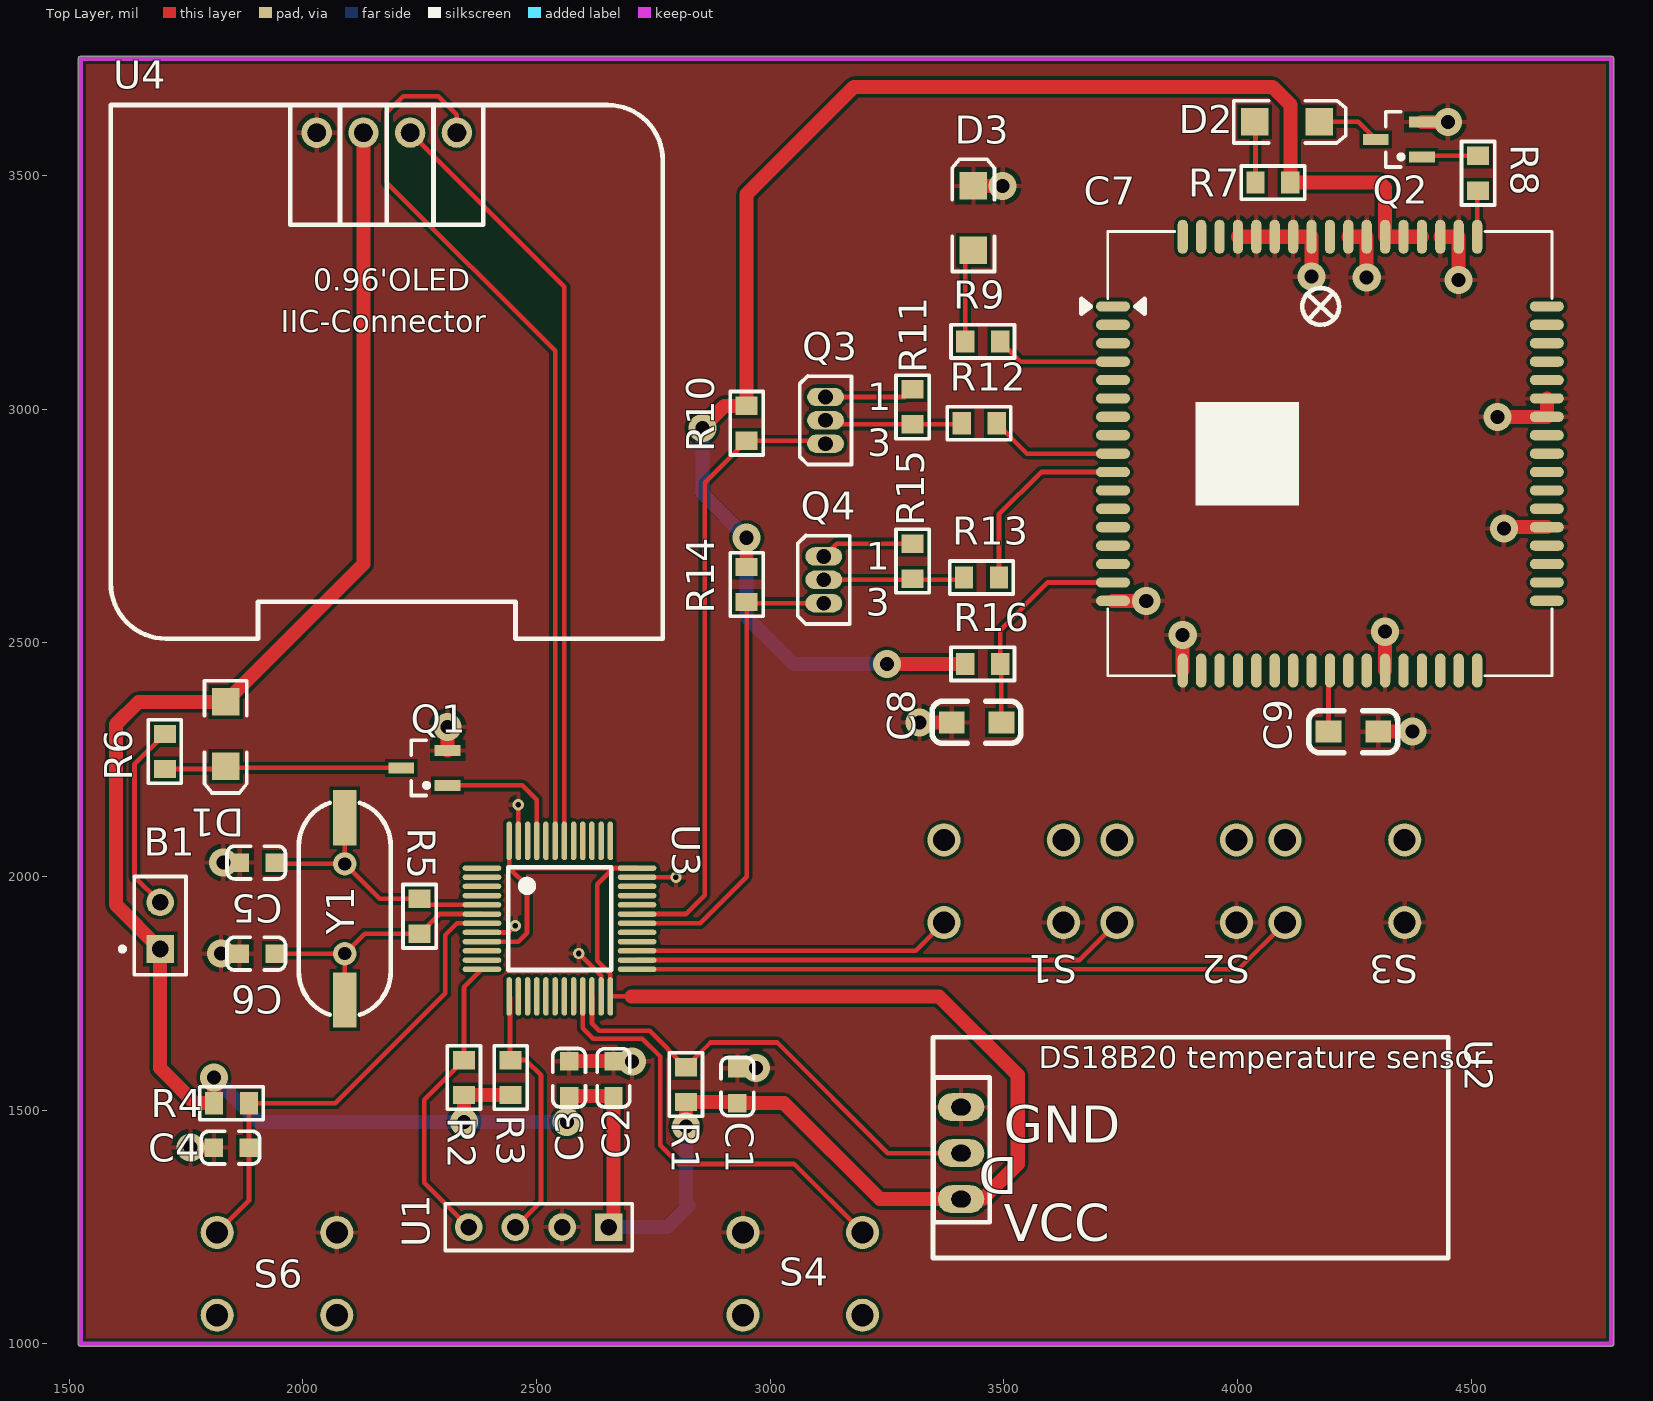
[diagram p0: Top Layer view]
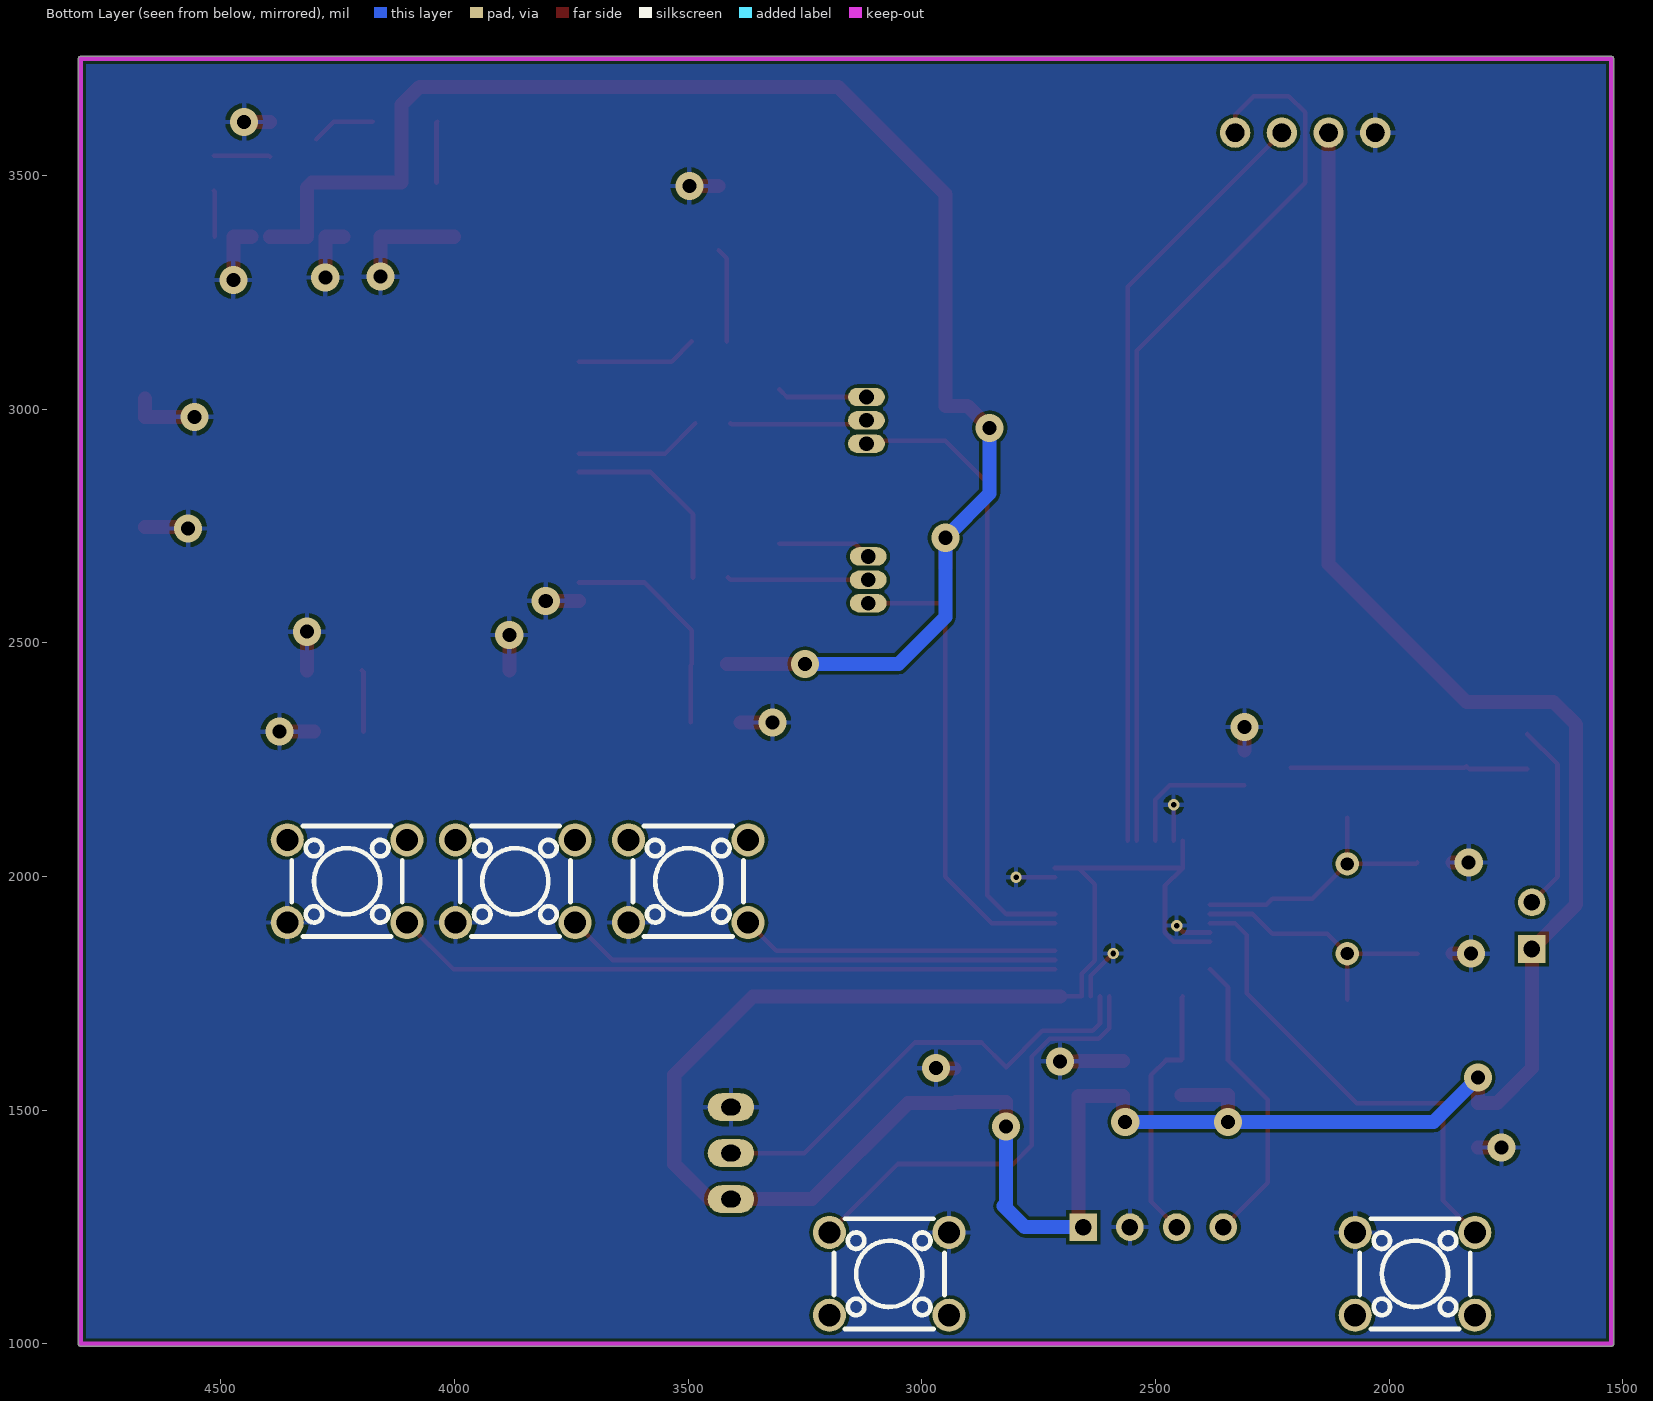
[diagram p1: Bottom Layer view, seen from below]
# Altium PCB MISC82701.PcbDoc
Units mil, origin at the board's own origin, x right, y up, seen from the top; angles counter-clockwise.
Board outline 3285.03 x 2760.03 mil, 2 copper layers (Top Layer, Bottom Layer); 43 components, 37 nets, 219 pads, 29 vias.

## Layer stack, top to bottom (the 12.6 mil dielectric is the usual default, probably not edited)
Top Solder: solder mask 0.4, Solder Resist, Dk 3.5
Top Layer: signal copper 1.4
Dielectric 1: dielectric 12.6, FR-4, Dk 4.8
Bottom Layer: signal copper 1.4
Bottom Solder: solder mask 0.4, Solder Resist, Dk 3.5

## Board outline
1519.98,1000 ccw(c1525,1000) 1525,994.99 4800,994.99 ccw(c4800,1000) 4805.02,1000 4805.02,3750 ccw(c4800,3750) 4800,3755.01 1525,3755.01 ccw(c1525,3750) 1519.98,3750

## Design rules (kind name [scope] priority, off if disabled: settings)
Clearance [All] p1: gap=7
MinimumSolderMaskSliver [All] p1: minsoldermaskwidth=0
PolygonConnect [All] p1: connectstyle=Relief reliefconductorwidth=10 reliefentries=4 polygonreliefangle="90 Angle" airgapwidth=10
RoutingVias [All] p1: holewidth=28 width=50 viastyle="Through Hole" minholewidth=28 minwidth=50 maxholewidth=28 maxwidth=50
SilkToSilkClearance [All] p1: silktosilkclearance=0
SilkToSolderMaskClearance [IsPad] p1: minsilkscreentomaskgap=0 clearancetoexposedcopper=TRUE
SolderMaskExpansion [All] p1: expansion=4
Width [All] p1: maxlimit=30 minlimit=10 preferedwidth=10
27 further rules are at their usual default settings.

## Components (designator, comment, footprint, x,y, rotation, side; value= is the part's Value field where it differs from the comment)
B1 "Buzzer" PIN2 1695,1845 r90 top
C1 "Capacitor" 0603C 2930,1589.8 r270 top
C2 "Capacitor" 0603C 2665,1530 r90 top
C3 "Capacitor" 0603C 2570,1530.2 r90 top
C4 "10uF" 0603C 1884.8,1420 r180 top
C5 "Cap" 0603C 1940,2030 r180 top
C6 "Cap" 0603C 1939.8,1835 r180 top
C7 "SIM800C GSM module" GSMM_SMD_SIM900A 4180,2905 r0 top
C8 "Capacitor" 0805C 3388.7,2330 r180 top
C9 "Capacitor" 0805C 4195,2310 r180 top
D1 "LED" 3.2X1.6X1.1 1835,2305 r270 top
D2 "LED" 3.2X1.6X1.1 4106.1,3615 r0 top
D3 "LED" 3.2X1.6X1.1 3435,3408.9 r90 top
Q1 "N-MOSFET" SOT23 2310,2195.2 r90 top
Q2 "N-MOSFET" SOT23 4395,3540 r90 top
Q3 "MOSFET P" E3 3118.73,2976.18 r0 top
Q4 "MOSFET P" E3 3115,2635 r0 top
R1 "Resistor" 0805R 2820,1555 r270 top
R2 "Resistor" 0805R 2345,1570 r270 top
R3 "Resistor" 0805R 2445,1570 r270 top
R4 "Res Semi" 0805R 1847.6,1515 r0 top
R5 "Res Semi" 0805R 2250,1915 r270 top
R6 "Resistor" 0805R 1705,2267.6 r90 top
R7 "Resistor" 0805R 4076.1,3485 r0 top
R8 "Resistor" 0805R 4515,3505 r270 top
R9 "Resistor" 0805R 3455,3145 r0 top
R10 "Resistor" 0805R 2950,2970 r90 top
R11 "Resistor" 0805R 3305,3005 r90 top
R12 "Resistor" 0805R 3447.4,2970 r0 top
R13 "Resistor" 0805R 3452.4,2640 r0 top
R14 "Resistor" 0805R 2950,2625 r90 top
R15 "Resistor" 0805R 3305,2675 r90 top
R16 "Resistor" 0805R 3455,2455 r0 top
S1 "Screen switch key" 四脚轻触开关 3500,1990 r180 top
S2 "Cursor switch key" 四脚轻触开关 3870,1990 r180 top
S3 "Value decrease key" 四脚轻触开关 4230,1990 r180 top
S4 "Value increase key" 四脚轻触开关 3070,1150 r0 top
S6 "Key" 四脚轻触开关 1945,1150 r0 top
U1 "ASR01 speech recognition module" HDR1X4 2655,1250 r180 top
U2 "DS18B20 temperature sensor" DS18B20 3900,1420 r0 top
U3 "STM32" "LQFP48 7X7" 2550,1910 r270 top
U4 "OLED display" 0.96OLED_4P 2180,3080 r0 top
Y1 "XTAL" XTAL_US 2090,1835 r90 top

## Footprints (in the part's own frame and the unit in brackets; to place one, negate y for a bottom-side part, rotate by r counter-clockwise, add the part's x,y. Pads: shape width x height; smd on the part's side, far side on the other; paste and mask are expansions set on the pad)
0.96OLED_4P [mm]
  round 1.65 hole 1 slot 1.005 at 0 deg paste+0 mask+0.051: 1(-3.811,12.997) 2(-1.271,13) 3(1.269,13) 4(3.809,13)
  silkscreen extent -15,-14.5 15,14.5
3.2X1.6X1.1 [mm] "SMT LED; 2 Flat Leads"
  rect 1.5x1.5 smd: 1(-1.75,0) 2(1.75,0)
  silkscreen extent -2.9,-1.15 3.2,1.15
0603C [mm]
  rect 1x1 smd: 1(0,0) 2(1.9,0)
  silkscreen extent -0.59,-0.89 2.59,0.89
0805C [mm]
  rect 1.4x1.2 smd: 1(0,0) 2(-2.7,0)
  silkscreen extent -3.76,-1.14 1.07,1.14
0805R [mm]
  rect 1x1.2 smd: 1(-0.95,0) 2(0.95,0)
  silkscreen extent -1.73,-0.9 1.73,0.9, body extent -1,-0.64 1,0.64, height 0.65
DS18B20 [mil]
  oval 99.37x60 hole 35.43 slot 41.34 at 0 deg paste+0 mask+4: 1(-491.35,86.55) 2(-491.35,-11.88) 3(-491.35,-110.3)
  silkscreen extent -551,-236 551,236
E3 [mm] "TO, Flat Index; 3 In-Line, Axial Leads; Body Dia. 4.6mm; Lead Dia. 0.5 mm (max)"
  oval 2x1 hole 0.8: 1(0,1.27) 2(0,0) 3(0,-1.27)
  silkscreen extent -1.41,-2.41 1.41,2.41
GSMM_SMD_SIM900A [mm]
  oval 1.85x0.56 smd paste+0 mask+0.051: 1(-11.331,8) 2(-11.331,7) 3(-11.331,6) 4(-11.331,5) 5(-11.331,4) 6(-11.331,3) 7(-11.331,2) 8(-11.331,1) 9(-11.331,0) 10(-11.331,-1) 11(-11.331,-2) 12(-11.331,-3) 13(-11.331,-4) 14(-11.331,-5) 15(-11.331,-6) 16(-11.331,-7) 17(-11.331,-8) 35(12.244,-8) 36(12.244,-7) 37(12.244,-6) 38(12.244,-5) 39(12.244,-4) 40(12.244,-3) 41(12.244,-2) 42(12.244,-1) 43(12.244,0) 44(12.244,1) 45(12.244,2) 46(12.244,3) 47(12.244,4) 48(12.244,5) 49(12.244,6) 50(12.244,7) 51(12.244,8)
  oval 0.56x1.85 smd paste+0 mask+0.051: 18(-7.543,-11.787) 19(-6.543,-11.787) 20(-5.543,-11.787) 21(-4.543,-11.787) 22(-3.543,-11.787) 23(-2.543,-11.787) 24(-1.543,-11.787) 25(-0.543,-11.787) 26(0.457,-11.787) 27(1.457,-11.787) 28(2.457,-11.787) 29(3.457,-11.787) 30(4.457,-11.787) 31(5.457,-11.787) 32(6.457,-11.787) 33(7.457,-11.787) 34(8.457,-11.787) 52(8.457,11.787) 53(7.457,11.787) 54(6.457,11.787) 55(5.457,11.787) 56(4.457,11.787) 57(3.457,11.787) 58(2.457,11.787) 59(1.457,11.787) 60(0.457,11.787) 61(-0.543,11.787) 62(-1.543,11.787) 63(-2.543,11.787) 64(-3.543,11.787) 65(-4.543,11.787) 66(-5.543,11.787) 67(-6.543,11.787) 68(-7.543,11.787)
  silkscreen extent -13.04,-12.08 12.53,12.08
HDR1X4 [mm] "Connector; Header; 4 Position"
  rect 1.5x1.5 hole 0.9: 1(0,0)
  round 1.5 hole 0.9: 2(2.54,0) 3(5.08,0) 4(7.62,0)
  silkscreen extent -1.27,-1.27 8.89,1.27
"LQFP48 7X7" [mm]
  oval 0.3x2.1 smd: 1(-2.75,-4.227) 2(-2.25,-4.227) 3(-1.75,-4.227) 4(-1.25,-4.227) 5(-0.75,-4.227) 6(-0.25,-4.227) 7(0.25,-4.227) 8(0.75,-4.227) 9(1.25,-4.227) 10(1.75,-4.227) 11(2.25,-4.227) 12(2.75,-4.227) 25(2.75,4.202) 26(2.25,4.202) 27(1.75,4.202) 28(1.25,4.202) 29(0.75,4.202) 30(0.25,4.202) 31(-0.25,4.202) 32(-0.75,4.202) 33(-1.25,4.202) 34(-1.75,4.202) 35(-2.25,4.202) 36(-2.75,4.202)
  oval 2.1x0.3 smd: 13(4.227,-2.75) 14(4.227,-2.25) 15(4.227,-1.75) 16(4.227,-1.25) 17(4.227,-0.75) 18(4.227,-0.25) 19(4.227,0.25) 20(4.227,0.75) 21(4.227,1.25) 22(4.227,1.75) 23(4.227,2.25) 24(4.227,2.75) 37(-4.227,2.75) 38(-4.227,2.25) 39(-4.227,1.75) 40(-4.227,1.25) 41(-4.227,0.75) 42(-4.227,0.25) 43(-4.227,-0.25) 44(-4.227,-0.75) 45(-4.227,-1.25) 46(-4.227,-1.75) 47(-4.227,-2.25) 48(-4.227,-2.75)
  silkscreen extent -2.79,-2.79 2.79,2.79, body extent -4.51,-4.5 4.5,4.5, height 1.45
PIN2 [mm] "Photosensitive Diode; 2 Leads"
  rect 1.5x1.5 hole 0.9: 1(0,0)
  round 1.5 hole 0.9: 2(2.54,0)
  silkscreen extent -1.4,-1.4 3.94,2.17
SOT23 [mm]
  rect 0.6x1.4 smd: D(0.95,2.514) G(0,0) S(1.9,0)
  silkscreen extent -0.55,1.02 2.45,1.97, body extent -0.56,0.22 2.44,2.62, height 1.05
XTAL_US [mm]
  rect 3x1.27 smd: 1(-2.51,0) 2(7.39,0)
  round 1.27 hole 0.711: 1(0,0) 2(4.88,0)
  silkscreen extent -3.33,-2.5 8.21,2.5
四脚轻触开关 [mm]
  round 1.8 hole 1.2 paste+0 mask+0.102: 1(3.25,2.25) 2(-3.25,2.25) 3(3.25,-2.25) 4(-3.25,-2.25)

## Part data
B1: library part 蜂鸣器
C1 C2 C3 C8 C9: library part 电容, "SMD capacitor"
C4: library part "Cap Semi", "Capacitor (Semiconductor SIM Model)"
C5 C6: "Capacitor"
C7: library part "SIM 900A"
D1 D2 D3: library part LED灯
Q1 Q2: library part SI2302, "MOSFET"
R1 R2 R3 R6 R7 R8 R9 R10 R11 R12 R13 R14 R15 R16: library part 电阻, "SMD resistor"
R4 R5: "Semiconductor Resistor"
S1 S2 S3 S4 S6: library part 按键
U1: library part HC-05蓝牙模块_1, "HC-05 Bluetooth module"
U2: library part DS18B20, "Temperature sensor"
U3: library part STM32F103C8T6_2
U4: library part OLED显示器2
Y1: "Crystal Oscillator"

## Via types
v1: diameter 60, hole 30, Top Layer to Bottom Layer, 25 vias
v2: diameter 24, hole 12, Top Layer to Bottom Layer, 4 vias

## Nets (pads, with @x,y where several pads share a name; then routed paths per layer and width w, separated by ;. In a path a pad name is that pad's centre, name@x,y a point inside that pad or via, vN(x,y) a via of type N, cw(c..) or ccw(c..) an arc to the next point about the centre after c; other vN are vias at no path point)
GND: C1.1 C2.2 C3.2 C4.2 C5.2 C6.2 C7.17 C7.18 C7.29 C7.39 C7.45 C7.46 C7.53 C7.54 C7.58 C7.59 C7.61 C7.62 C7.63 C7.64 C7.65 C8.1 C9.2 D3.2 Q1.S Q2.S S1.2 S2.2 S3.2 S4.2 S6.1 U1.2 U2.1 U3.8 U3.23 U3.35 U3.47 U4.1 | length 1931.4
  Top Layer w10: U3.8 2440.47,1880.47 v2(2455,1895) ; U3.47 v2(2461.42,2153.58) ; v2(2590.48,1835.48) 2638.58,1787.38 U3.23 ; U3.35 v2(2798.58,1998.58)
  Top Layer w30: v1(1760,1420) C4.2 ; v1(1825,1835) C6.2 ; v1(1830,2030) C5.2 ; Q1.S v1(2310,2320) ; C3.2 2664.8,1605 C2.2 v1(2704.8,1604.8) ; C1.1 v1@2979.8,1589.8 ; v1(3320,2330) C8.1 ; D3.2 v1(3497.8,3477.8) ; C7.17 v1(3804.96,2590.04) ; C7.18 v1(3883.03,2516.97) ; C7.65 C7.64 C7.63 C7.62 C7.61 v1(4158.62,3283.62) ; C7.59 C7.58 v1(4276.73,3281.73) ; C9.2 v1(4375,2310) ; C7.29 v1(4316.1,2523.9) ; Q2.S v1(4450.2,3614.8) ; C7.54 C7.53 v1(4473.58,3276.42) ; v1(4556.26,2983.74) C7.45 C7.46 ; v1@4577.48,2747.52 C7.39
  other v1: 2970,1590 4570,2745
NetB1_2: B1.2 R6.2 | length 409.7
  Top Layer w10: B1.2 1640,2000 1640,2240 R6.2
NetC4_1: C4.1 R4.2 S6.2 U3.7 | length 1035.9
  Top Layer w10: S6.2 1885,1306.54 R4.2 2070,1515 2305,1750 2305,1875 2330.16,1900.16 U3.7
NetC5_1: C5.1 R5.1 U3.5 Y1.2 | length 579.9
  Top Layer w10: C5.1 1942.87,2027.13 Y1.2@2090,2027.13 ; Y1.2@2090,2125.94 Y1.2@2090,2027.13 ; U3.5 2262.87,1939.53 R5.1 2164.72,1952.4 Y1.2@2090,2027.13
NetC6_1: C6.1 R5.2 U3.6 Y1.1 | length 577.7
  Top Layer w10: C6.1 Y1.1@2090,1835 ; Y1.1@2090,1736.18 Y1.1@2090,1835 ; U3.6 2292.24,1919.84 R5.2 2132.6,1877.6 Y1.1@2090,1835
NetC7_4: C7.4 R9.2 | length 259.4
  Top Layer w10: R9.2 3535.55,3101.85 C7.4
NetC7_9: C7.9 R12.2 | length 276
  Top Layer w10: R12.2 3549.8,2905 C7.9
NetC7_10: C7.10 R13.2 | length 416.5
  Top Layer w10: R13.2 3489.8,2774.8 3580.63,2865.63 C7.10
NetC7_16: C7.16 C8.2 R16.2 | length 482.2
  Top Layer w10: C8.2 3495,2452.4 R16.2 3492.4,2527.4 3594.41,2629.41 C7.16
NetC7_26: C7.26 C9.1 | length 132.2
  Top Layer w10: C9.1 4195,2437.94 C7.26
NetC7_52: C7.52 R8.2 | length 99.4
  Top Layer w10: C7.52 4512.95,3465.55 R8.2
NetD1_2: D1.2 Q1.D R6.1 | length 509.9
  Top Layer w10: R6.1 1829.09,2230.2 D1.2 1838.5,2232.6 Q1.D
NetD2_1: D2.1 R7.1 | length 130.6
  Top Layer w10: D2.1 4038.7,3613.5 R7.1
NetD2_2: D2.2 Q2.D | length 136.6
  Top Layer w10: D2.2 4258.43,3615 Q2.D
NetD3_1: D3.1 R9.1 | length 202.2
  Top Layer w10: R9.1 3417.6,3322.6 D3.1
NetQ1_1: Q1.G U3.45 | length 291.4
  Top Layer w10: Q1.G 2469.8,2195.2 2500.79,2164.21 U3.45
NetQ2_1: Q2.G R8.1 | length 121
  Top Layer w10: Q2.G 4397.4,3542.4 R8.1
NetQ3_1: Q3.1 R11.2 | length 193
  Top Layer w10: Q3.1 3288.78,3026.18 R11.2
NetQ4_1: Q4.1 R15.2 | length 201.4
  Top Layer w10: Q4.1 3142.4,2712.4 R15.2
NetR1_1: R1.1 U2.2 U3.22 | length 1006
  Top Layer w10: U3.22 2618.9,1686.1 2635,1670 2742.4,1670 R1.1 2872.6,1645 3015,1645 3251.88,1408.12 U2.2
NetR2_1: R2.1 U1.4 U3.12 | length 642.3
  Top Layer w10: U1.4 2260,1345 2260,1522.4 R2.1 2345,1763.15 U3.12
NetR3_1: R3.1 U1.3 U3.13 | length 563.7
  Top Layer w10: U3.13 2443.51,1741.8 2443.51,1608.89 R3.1 2477.6,1607.4 2510,1575 2510,1305 U1.3
NetS1_1: S1.1 U3.27 | length 681.6
  Top Layer w10: U3.27 3311.73,1841.1 S1.1
NetS2_1: S2.1 U3.26 | length 1059.8
  Top Layer w10: U3.26 3662.05,1821.42 S2.1
NetS3_1: S3.1 U3.25 | length 1427.9
  Top Layer w10: U3.25 4002.36,1801.73 S3.1
NetS4_1: S4.1 U3.21 | length 958.9
  Top Layer w10: U3.21 2599.21,1675.79 2622,1653 2727,1653 2765,1615 2765,1425 2805,1385 3051.54,1385 S4.1
NetU3_42: U3.42 U4.3 | length 1652
  Top Layer w10: U4.3 2559.84,3261.91 U3.42
NetU3_43: U3.43 U4.4 | length 1927
  Top Layer w10: U4.4 2329.95,3630.05 2290,3670 2215,3670 2180,3635 2180,3485 2540.16,3124.84 U3.43
POWKEY: C7.1
RF: C7.60
RXD: Q4.3 R14.1 U3.30 | length 1023
  Top Layer w10: U3.30 2850.16,1900.16 2950,2000 2950,2580 2955,2585 Q4.3
SIM_RXD: Q4.2 R13.1 R15.1 | length 302.1
  Top Layer w10: Q4.2 3410,2635 R13.1
SIM_TXD: Q3.2 R11.1 R12.1 | length 295.8
  Top Layer w10: Q3.2 3127.31,2967.6 R11.1 3407.6,2967.6 R12.1
TXD: Q3.3 R10.1 U3.31 | length 1342.5
  Top Layer w10: U3.31 2819.84,1919.84 2860,1960 2860,2842.6 R10.1 3112.31,2932.6 Q3.3
VCC: B1.1 C1.2 C2.1 C3.1 D1.1 R1.2 R2.2 R3.2 R4.1 U1.1 U2.3 U3.9 U3.24 U3.36 U3.48 U4.2 | length 7222.4
  Top Layer w10: U3.9 2460.79,1860.79 2480,1880 2480,1980 2441.73,2018.27 ; U3.48 2441.73,2018.27 ; 2703.58,1743.58 U3.24 2658.27,1791.73 2630,1820 2630,1983.71 2664.56,2018.27 ; U3.36 2664.56,2018.27 ; 2441.73,2018.27 2664.56,2018.27
  Top Layer w30: v1@1810,1570 v1(1810.2,1569.8) R4.1 1770,1515 1695,1590 B1.1 1600,1940 1600,2325 1648.9,2373.9 D1.1 2129.95,2668.85 U4.2 ; v1(2345,1475) R2.2 R3.2 ; v1(2565,1475) 2570,1480 C3.1 2664.8,1530.2 C2.1 2665,1260 U1.1 ; 2703.58,1743.58 3361.42,1743.58 3530,1575 3530,1385 3454.7,1309.7 U2.3 3235.3,1309.7 3030,1515 C1.2 2927.4,1517.6 R1.2 v1(2820,1465)
  Bottom Layer w30: v1(1810.2,1569.8) 1905,1475 v1(2345,1475) v1(2565,1475) ; U1.1 2780,1250 2825,1295 2820,1300 v1(2820,1465)
VCC_4: C7.55 C7.56 C7.57 R7.2 R10.2 R14.2 R16.1 | length 3425.2
  Top Layer w30: v1(2855,2960) 2902.4,3007.4 R10.2 2950,3460 3180,3690 4075,3690 4113.5,3651.5 R7.2 4305,3485 4316.1,3473.9 C7.57 C7.56 C7.55 ; R14.2 v1(2950,2725) ; v1(3250,2455) R16.1
  Bottom Layer w30: v1@2855,2970 v1(2855,2960) 2855,2820 v1(2950,2725) 2950,2555 3050,2455 v1(3250,2455)
VDD_EXT: C7.15
pads on no net: C7.2 C7.3 C7.5 C7.6 C7.7 C7.8 C7.11 C7.12 C7.13 C7.14 C7.19 C7.20 C7.21 C7.22 C7.23 C7.24 C7.25 C7.27 C7.28 C7.30 C7.31 C7.32 C7.33 C7.34 C7.35 C7.36 C7.37 C7.38 C7.40 C7.41 C7.42 C7.43 C7.44 C7.47 C7.48 C7.49 C7.50 C7.51 C7.66 C7.67 C7.68 S1.3 S1.4 S2.3 S2.4 S3.3 S3.4 S4.3 S4.4 S6.3 S6.4 U3.1 U3.2 U3.3 U3.4 U3.10 U3.11 U3.14 U3.15 U3.16 U3.17 U3.18 U3.19 U3.20 U3.28 U3.29 U3.32 U3.33 U3.34 U3.37 U3.38 U3.39 U3.40 U3.41 U3.44 U3.46

## Polygon pours and split planes (outlines as drawn)
GND on Top Layer "G" (solid, remove dead copper, pour order 0): 1085,3875 1095,3885 4955,3885 4955,890 4920,855 4895,880 1215,880
GND on Bottom Layer "G" (solid, remove dead copper, pour order 2): 1400,3855 4950,3855 4965,3840 4910,3785 4910,840 1510,840 1435,765

## Keep-outs
Keep-Out Layer:
  lines w10: 4265,3750 4800,3750 4800,1000 1525,1000 1525,3750 4325,3750